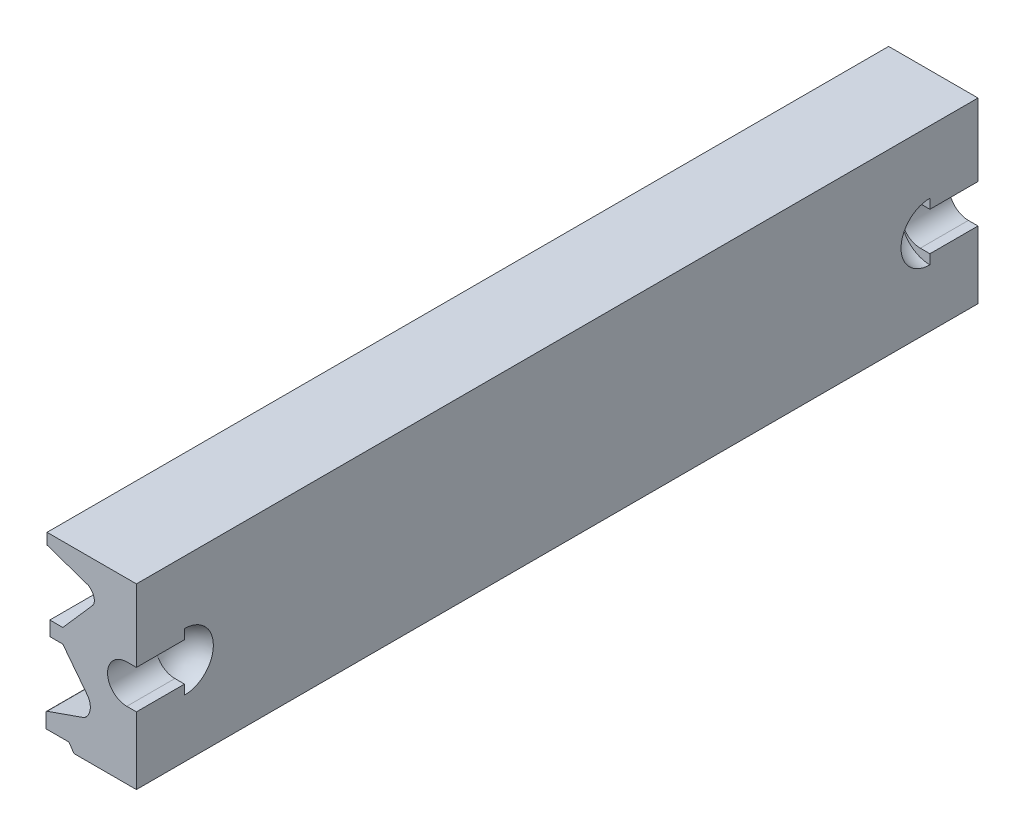
SolidWorks part; units mm, degrees
ref_plane "前视基准面" through (0, 0, 0) normal (0, 0, 1) x (1, 0, 0)
ref_plane "上视基准面" through (0, 0, 0) normal (0, 1, 0) x (1, 0, 0)
ref_plane "右视基准面" through (0, 0, 0) normal (1, 0, 0) x (0, 0, -1)
sketch "草图1" plane through (0, 0, 0) normal (0, 0, 1) x (1, 0, 0)
  line L0 (0, -144.6383) -> (-130, -144.6383)
  line L1 (-130, -144.6383) -> (-140.2996, -129.1889)
  line L14 (0, 185.6971) -> (0, 75.8111)
  line L16 (0, -144.6383) -> (0, -4.1889)
  line L18 (-187.997, -129.1889) -> (-187.997, -99.1889)
  line L23 (-140.2996, -129.1889) -> (-187.997, -129.1889)
  line L30 (-153.0142, 40.8148) -> (-180.0142, 40.8148)
  line L31 (-180.0142, 40.8148) -> (-180.0142, 70.8148)
  line L33 (-102.3154, -24.8968) -> (-153.0142, 40.8148)
  line L35 (-180.0142, 70.8148) -> (-153.0142, 70.8148)
  line L46 (-185.8039, -96.424) -> (-108.027, -69.1852)
  line L52 (181.9161, 650.8148) -> (206.9161, 650.8148)
  line L55 (-185.8039, 202.8148) -> (-100.0142, 173.2895)
  line L56 (0, 75.8111) -> (0, -4.1889)
  line L58 (-92.1921, 140.123) -> (-153.0142, 70.8148)
  line L59 (-108.0839, 225.8148) -> (-185.8039, 225.8148)
  line L60 (-185.8039, 225.8148) -> (-185.8039, 202.8148)
  line L61 (0, 185.6971) -> (0, 225.8148)
  line L62 (0, 225.8148) -> (-108.0839, 225.8148)
  arc A4 (-108.027, -69.1852) -> (-102.3154, -24.8968) centre (-127.3154, -44.1852) ccw
  spline S0 degree 2 poles (-187.997, -99.1889) (-187.7382, -97.2424) (-185.8039, -96.424) knots 0 0 0 1 1 1
  spline S1 degree 3 poles (-100.0142, 173.2895) (-89.2423, 167.1735) (-82.4916, 150.1954) (-92.1921, 140.123) knots 0 0 0 0 1 1 1 1
extrude "凸台-拉伸1" add sketch "草图1" against normal blind 1750
sketch "草图3" plane through (0, 0, 0) normal (0, 0, 1) x (1, 0, 0)
  line L1 (0, -144.6383) -> (0, 225.8148) construction
  line L2 (0, -4.6383) -> (-20, -4.6383)
  line L3 (-20, 75.3617) -> (0, 75.3617)
  line L4 (0, 75.3617) -> (0, -4.6383)
  arc A0 (-20, -4.6383) -> (-20, 75.3617) centre (-20, 35.3617) cw
extrude "切除-拉伸3" cut sketch "草图3" against normal blind 100
sketch3d "3D草图2"
  point P0 (0, 60.7879, -290.1209)
ref_plane "基准面3" through (0, 0, 0) normal (1, 0, 0) x (0, 0, -1)
sketch "草图5" plane through (0, 0, 0) normal (1, 0, 0) x (0, 0, -1)
  line L0 (100, 95.3617) -> (100, -24.6383)
  line L1 (100, 75.3617) -> (100, -4.6383) construction
  arc A0 (100, 95.3617) -> (100, -24.6383) centre (100, 35.3617) cw
revolve "切除-旋转1" cut sketch "草图5" angle 90 about L0
ref_plane "基准面4" through (0, 0, -875) normal (0, 0, 1) x (1, 0, 0)
mirror "镜向1" about plane through (0, 0, -875) normal (0, 0, 1) of "切除-拉伸3", "切除-旋转1"
